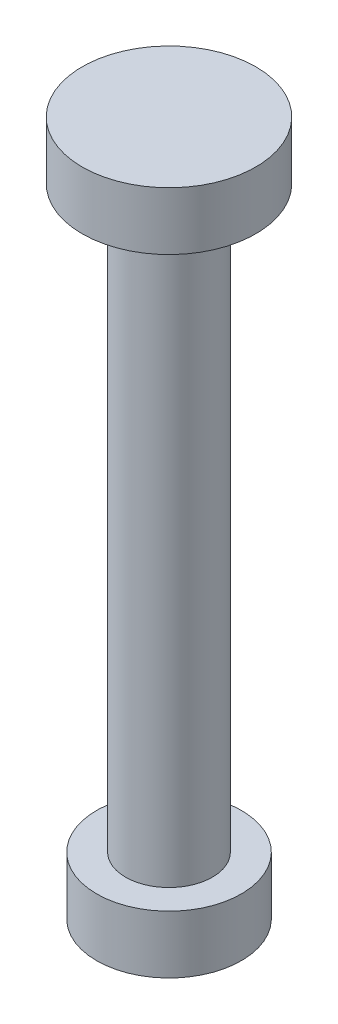
SolidWorks part; units mm, degrees
ref_plane "Front Plane" through (0, 0, 0) normal (0, 0, 1) x (1, 0, 0)
ref_plane "Top Plane" through (0, 0, 0) normal (0, 1, 0) x (1, 0, 0)
ref_plane "Right Plane" through (0, 0, 0) normal (1, 0, 0) x (0, 0, -1)
other "Configuration Table"
sketch "Sketch1" plane through (0, 0, 0) normal (0, 0, 1) x (1, 0, 0)
  line L0 (0, 0) -> (2.5, 0)
  line L1 (2.5, 0) -> (2.5, 2)
  line L2 (2.5, 2) -> (1.5, 2)
  line L3 (1.5, 2) -> (1.5, 22)
  line L4 (1.5, 22) -> (3, 22)
  line L5 (3, 22) -> (3, 24)
  line L6 (3, 24) -> (0, 24)
  line L7 (0, 24) -> (0, 0)
  dimension "D1" = 2.5
  dimension "D2" = 2
  dimension "D3" = 20
  dimension "D4" = 2
  dimension "D5" = 1.5
  dimension "D6" = 1.5
revolve "Revolve1" add sketch "Sketch1" angle 360 about L7
